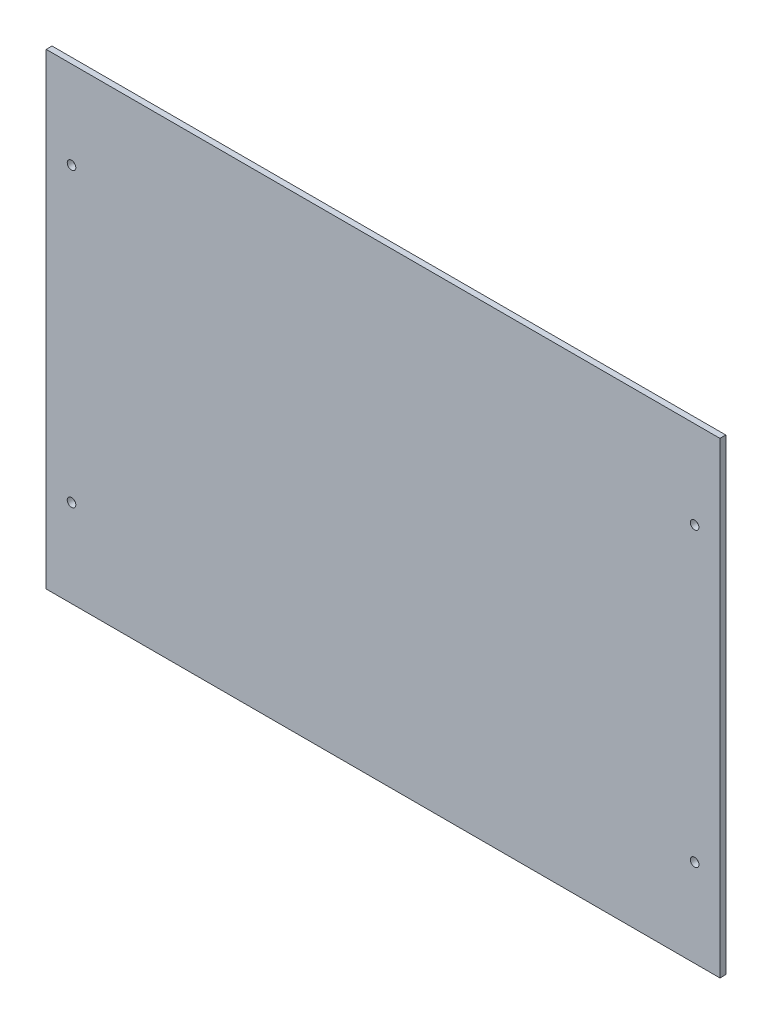
SolidWorks part; units mm, degrees
ref_plane "前视基准面" through (0, 0, 0) normal (0, 0, 1) x (1, 0, 0)
ref_plane "上视基准面" through (0, 0, 0) normal (0, 1, 0) x (1, 0, 0)
ref_plane "右视基准面" through (0, 0, 0) normal (1, 0, 0) x (0, 0, -1)
sketch "草图1" plane through (0, 0, 0) normal (0, 0, 1) x (1, 0, 0)
  line L1 (173, -120) -> (-173, -120)
  line L2 (173, -120) -> (173, 120)
  line L3 (173, 120) -> (-173, 120)
  line L4 (-173, -120) -> (-173, 120)
  line L5 (173, -120) -> (-173, 120) construction
  line L6 (173, 120) -> (-173, -120) construction
  point P0 (0, 0)
  dimension "D1" = 346
  dimension "D2" = 240
extrude "凸台-拉伸1" add sketch "草图1" along normal blind 3
sketch "草图2" plane through (0, 0, 3) normal (0, 0, 1) x (1, 0, 0)
  line L0 (173, -120) -> (173, 120) construction
  line L1 (160, -75) -> (-160, -75) construction
  line L2 (160, -75) -> (160, 75) construction
  line L3 (160, 75) -> (-160, 75) construction
  line L4 (-160, -75) -> (-160, 75) construction
  line L5 (160, -75) -> (-160, 75) construction
  line L6 (160, 75) -> (-160, -75) construction
  circle A0 centre (160, 75) radius 2.2
  circle A1 centre (160, -75) radius 2.2
  circle A2 centre (-160, 75) radius 2.2
  circle A3 centre (-160, -75) radius 2.2
  circle A5 centre (-199.41, 140.4325) radius 2.2
  circle A6 centre (-199.41, -9.5675) radius 2.2
  point P0 (0, 0)
  dimension "D3" = 4.4
  dimension "D1" = 13
  dimension "D2" = 150
extrude "切除-拉伸1" cut sketch "草图2" against normal blind 10
